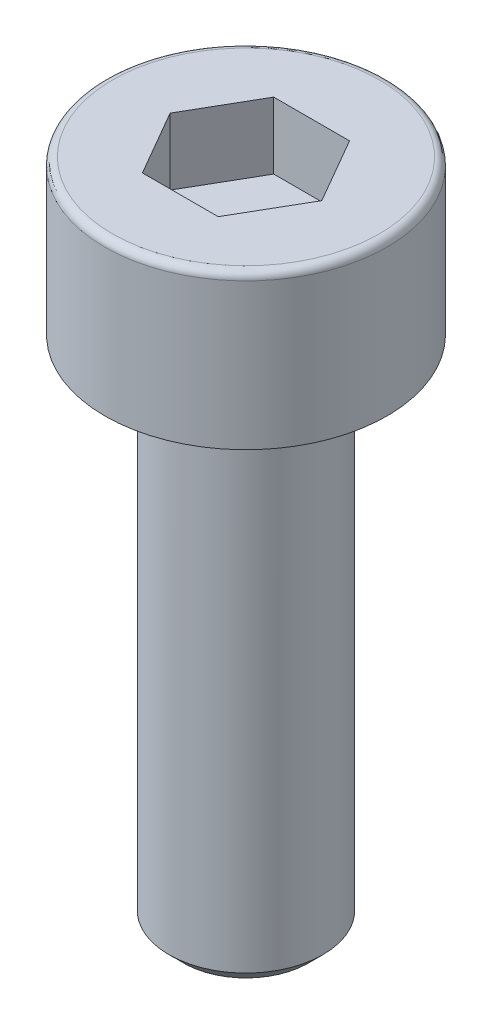
from build123d import *

# Parameters (mm, degrees)
SKETCH_1_R          = 2.75
EXTRUDE_1_DEPTH     = 3
CUT_EXTRUDE_1_DEPTH = 1.3
FILLET_1_R          = 0.15
SKETCH_5_R          = 1.5
EXTRUDE_2_DEPTH     = 10
CHAMFER_2_SIZE      = 0.28


with BuildPart() as part:
    # 草图1 → 凸台-拉伸1 (new body)
    with BuildSketch(Plane(origin=(0, 0, 0), x_dir=(1, 0, 0), z_dir=(0, 1, 0))):
        with Locations(Location((0, 0, 0), (0, 0, 270))):
            Circle(SKETCH_1_R)
    extrude(amount=EXTRUDE_1_DEPTH)

    # 草图2 → 切除-拉伸1 (cut)
    with BuildSketch(Plane(origin=(0, 3, 0), x_dir=(1, 0, 0), z_dir=(0, 1, 0))):
        Polygon((1.478016689, 0), (0.739008345, 1.28), (-0.739008345, 1.28), (-1.478016689, 0), (-0.739008345, -1.28), (0.739008345, -1.28), align=None)
    extrude(amount=-CUT_EXTRUDE_1_DEPTH, mode=Mode.SUBTRACT)

    # 圆角1
    fillet_1_edges = [part.edges().sort_by_distance(p)[0] for p in [
        (0, 3, -2.75),
    ]]
    fillet(fillet_1_edges, radius=FILLET_1_R)

    # 草图5 → 凸台-拉伸2 (add)
    with BuildSketch(Plane.XZ):
        with Locations(Location((0, 0, 0), (0, 0, 90))):
            Circle(SKETCH_5_R)
    extrude(amount=EXTRUDE_2_DEPTH)

    # 倒角2
    chamfer_2_edges = [part.edges().sort_by_distance(p)[0] for p in [
        (0, -10, -1.5),
    ]]
    chamfer(chamfer_2_edges, length=CHAMFER_2_SIZE)


solid = part.part
